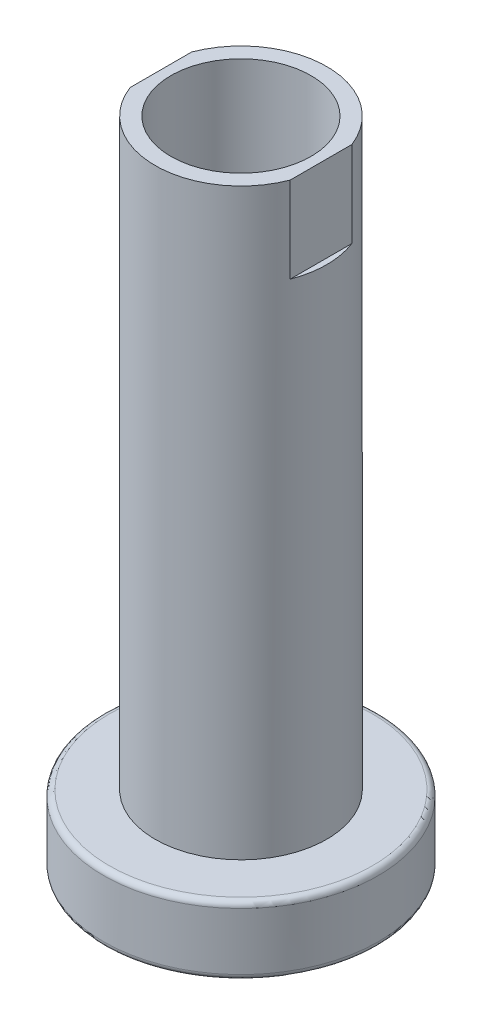
SolidWorks part; units mm, degrees
ref_plane "Front Plane" through (0, 0, 0) normal (0, 0, 1) x (1, 0, 0)
ref_plane "Top Plane" through (0, 0, 0) normal (0, 1, 0) x (1, 0, 0)
ref_plane "Right Plane" through (0, 0, 0) normal (1, 0, 0) x (0, 0, -1)
sketch "Sketch1" plane through (0, 0, 0) normal (0, 0, 1) x (1, 0, 0)
  line L0 (0, 92.0527) -> (0, -21.9473)
  line L1 (0, -21.9473) -> (-24, -21.9473)
  line L2 (-24, -21.9473) -> (-24, -9.9473)
  line L3 (-24, -9.9473) -> (-15, -9.9473)
  line L4 (-15, -9.9473) -> (-15, 92.0527)
  line L5 (-15, 92.0527) -> (0, 92.0527)
  dimension "D1" = 24
  dimension "D2" = 12
  dimension "D3" = 15
  dimension "D4" = 114
revolve "Revolve1" add sketch "Sketch1" angle 360 about L0
sketch "Sketch2" plane through (0, 0, 0) normal (0, 0, 1) x (1, 0, 0)
  line L0 (0, 111.6239) -> (0, 23.01) construction
  line L1 (14, 92.0527) -> (14, 77.0527)
  line L2 (-15, 92.0527) -> (-14, 92.0527)
  line L3 (-15, 92.0527) -> (-15, 77.0527)
  line L4 (-15, 77.0527) -> (-14, 77.0527)
  line L5 (-14, 92.0527) -> (-14, 77.0527)
  line L6 (15, 77.0527) -> (14, 77.0527)
  line L7 (15, 92.0527) -> (15, 77.0527)
  line L8 (15, 92.0527) -> (14, 92.0527)
  dimension "D1" = 14
  dimension "D2" = 15
extrude "Cut-Extrude1" cut sketch "Sketch2" against normal through all both and the other way through all
fillet "Fillet1" radius 1 2 edges at (-24, -21.9473, 0) (-24, -9.9473, 0)
hole_wizard "M27 Tapped Hole1" positions "Sketch3" profile "Sketch4" tap size "M27" standard "GB"
sketch "Sketch3" plane through (0, 92.0527, 0) normal (0, 1, 0) x (1, 0, 0)
  point P0 (0, 0)
sketch "Sketch4" plane through (0, 92.0527, 0) normal (1, 0, 0) x (0, 0, 1)
  line L0 (0, 0) -> (0, 43.3605)
  line L1 (0, 43.3605) -> (12.25, 36)
  line L2 (12.25, 36) -> (12.25, 0)
  line L5 (12.25, 0) -> (0, 0)
  line L10 (0, 43.3605) -> (-12.25, 36) construction
  line L11 (0, -6.35) -> (0, 107.95) construction
  dimension "螺纹孔钻头直径" = 24.5
  dimension "螺纹孔钻头深度" = 36
  dimension "导头角度" = 118
cosmetic thread "Cosmetic thread 1" parameters "D1"=36, "D2"=27
hole_wizard "M10 Tapped Hole1" positions "Sketch7" profile "Sketch6" tap size "M10" standard "GB"
sketch "Sketch7" plane through (0, -21.9473, 0) normal (0, -1, 0) x (-1, 0, 0)
  point P0 (0, 0)
sketch "Sketch6" plane through (0, -21.9473, 0) normal (1, 0, 0) x (0, 0, -1)
  line L0 (0, 0) -> (0, 22.5537)
  line L1 (0, 22.5537) -> (4.25, 20)
  line L2 (4.25, 20) -> (4.25, 0)
  line L5 (4.25, 0) -> (0, 0)
  line L10 (0, 22.5537) -> (-4.25, 20) construction
  line L11 (0, -6.35) -> (0, 107.95) construction
  dimension "螺纹孔钻头直径" = 8.5
  dimension "螺纹孔钻头深度" = 20
  dimension "导头角度" = 118
cosmetic thread "Cosmetic thread 2" parameters "D1"=20, "D2"=10
